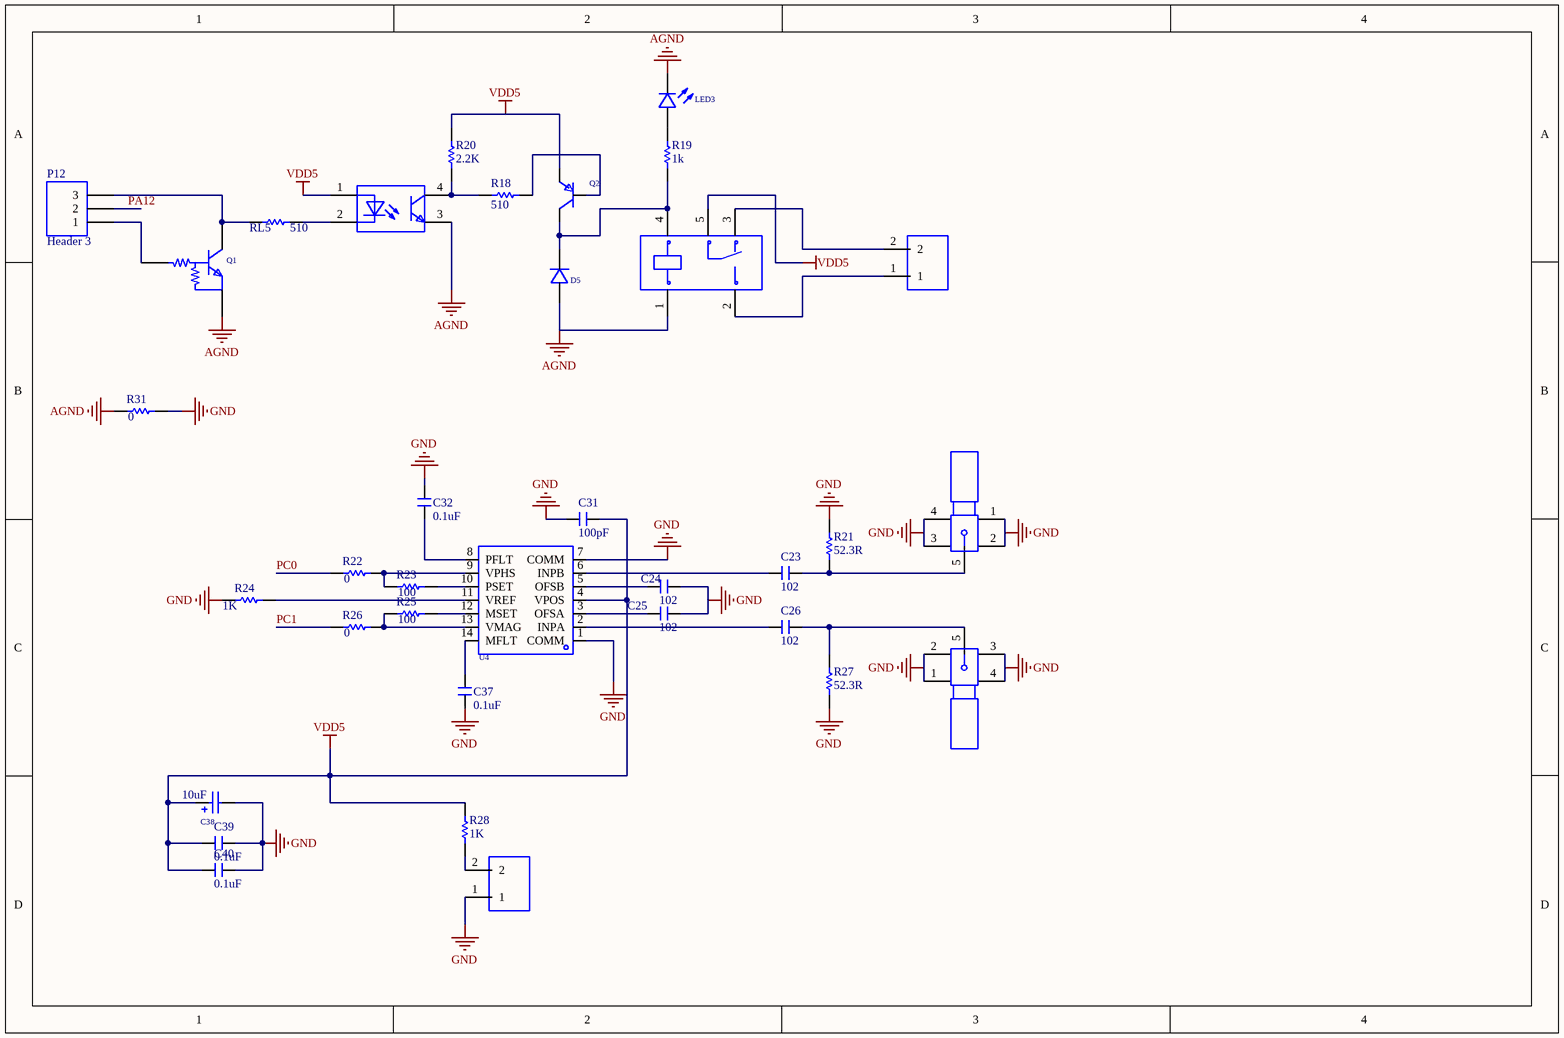
[diagram p0: MISC51485-4.schdoc]
# Altium project MISC51485-2.PrjPcb (part 1 of 2)
2 sheets, 98 parts. Net scope: global (net labels, ports and power ports of the same name join across sheets).
Board file: MISC51485.pcbdoc
Sheets:
  MISC51485-4.schdoc
  MISC51485-3.schdoc

## Sheet MISC51485-4.schdoc
size 292 x 193 mm; Device: *_1; SheetNumber: 2; SheetTotal: 2; Name: MISC51485

### Parts
C23  102  [C0603]
C24  102  [C0603]
C25  102  [C0603]
C26  102  [C0603]
C31  100pF  [C0603]
C32  0.1uF  [C0603]
C37  0.1uF  [C0603]
C38  10uF  [CAP-SMD_L3.2-W1.6-RD-C7171]
C39  0.1uF  [C0603]
C40  0.1uF  [C0603]
D5  1N4007W  [SOD-123FL_L2.7-W1.8-LS3.8-RD]  (value not drawn)
LED3  NCD0603R1_C84263  [LED0603-RD_RED]  (value not drawn)
P12  Header 3  [HDR1X3]
P13  WJ126V-5.0-2P  [CONN-TH_WJ126V-5.0-2P]  (value not drawn)
P17  WJ126V-5.0-2P  [CONN-TH_WJ126V-5.0-2P]  (value not drawn)
Q1  DTC143ECA  [SOT-23-3_L2.9-W1.6-P1.90-LS2.8-BR]  (value not drawn)
Q2  MMBT3906  [SOT-23-3_L2.9-W1.3-P1.90-LS2.4-BR]  (value not drawn)
R18  10k  [R0603 - duplicate]  (value not drawn)
R19  10k  [R0603 - duplicate]  (value not drawn)
R20  10k  [R0603 - duplicate]  (value not drawn)
R21  52.3R  [R0603]
R22  0  [R0603]
R23  100  [R0603]
R24  1K  [R0603]
R25  100  [R0603]
R26  0  [R0603]
R27  52.3R  [R0603]
R28  1K  [R0603]
R31  0  [R0603]
RF1  BWSMA-KWE-Z001  [SMA-TH_BWSMA-KWE-Z001]  (value not drawn)
RF?1  BWSMA-KWE-Z001  [SMA-TH_BWSMA-KWE-Z001]  (value not drawn)
RL5  330  [R0603 - duplicate]  (value not drawn)
RLY1  SRD-05VDC-SL-C  [RELAY-TH_SRD-XXVDC-XL-C]  (value not drawn)
U4  AD8302ARUZ-RL7  [TSSOP-14_L5.0-W4.4-P0.65-LS6.4-BL]  (value not drawn)
U6  BPC-817SC  [OPTO-SMD-4_L4.6-W6.5-P2.54-LS10.3-BR]  (value not drawn)

### Nets
AGND: D5.2(A) LED3.1(K) Q1.2(E) R31.1 RLY1.1 U6.3
GND: C24.1 C25.1 C31.2 C32.2 C37.1 C38.2 C39.1 C40.1 P17.1 R21.2 R24.1 R27.1 R31.2 RF1.1 RF1.2 RF1.3 RF1.4 RF?1.1 RF?1.2 RF?1.3 RF?1.4 U4.1(COMM) U4.7(COMM)
VDD5: C31.1 C38.1 C39.2 C40.2 Q2.2(E) R20.1 R28.2 RLY1.5 U4.4(VPOS) U6.1
PA12: P12.2
PC0: R22.1
PC1: R26.1
NetC23_1: C23.1 R21.1 RF1.5
NetC23_2: C23.2 U4.6(INPB)
NetC24_2: C24.2 U4.5(OFSB)
NetC25_2: C25.2 U4.3(OFSA)
NetC26_1: C26.1 R27.2 RF?1.5
NetC26_2: C26.2 U4.2(INPA)
NetC32_1: C32.1 U4.8(PFLT)
NetC37_2: C37.2 U4.14(MFLT)
NetD5_1: D5.1(K) Q2.3(C) R19.2 RLY1.4
NetLED3_2: LED3.2(A) R19.1
NetP12_1: P12.1 Q1.1(B)
NetP12_3: P12.3 Q1.3(C) RL5.1
NetP13_1: P13.1 RLY1.2
NetP13_2: P13.2 RLY1.3
NetP17_2: P17.2 R28.1
NetQ2_1: Q2.1(B) R18.2
NetR18_1: R18.1 R20.2 U6.4
NetR22_2: R22.2 R23.1 U4.9(VPHS)
NetR23_2: R23.2 U4.10(PSET)
NetR24_2: R24.2 U4.11(VREF)
NetR25_1: R25.1 R26.2 U4.13(VMAG)
NetR25_2: R25.2 U4.12(MSET)
NetRL5_2: RL5.2 U6.2

### Library data of the parts
C23 = 102: BOM名称: 无极性贴片电容; Origin Footprint: C 0201_L; OriginFootprint 2: C 0402_L; OriginFootprint 3: C 0603_L; OriginFootprint 4: C 0805_L; OriginFootprint 5: C 1206_L; OriginFootprint 6: C 1210_L; OriginFootprint 7: C 1808_L; OriginFootprint 8: C 1812_L; OriginFootprint 9: C 1825_L; OriginFootprint 10: C 2225_L; OriginFootprint 11: C 0201_M; OriginFootprint 12: C 0402_M; OriginFootprint 13: C 0603_M; OriginFootprint 14: C 0805_M; OriginFootprint 15: C 1206_M; OriginFootprint 16: C 1210_M; OriginFootprint 17: C 1808_M; OriginFootprint 18: C 1812_M; OriginFootprint 19: C 1825_M; OriginFootprint 20: C 2225_M; UniqueId: a6f4b5c625a68d3b; SymbolName: C; AddInBom: yes; ModelId: fca5be93b99f4b5a9a2fd372d58c31d9; Device: 102; DesignItemID: C; LibraryName: 3.1   - 电阻-电容-电感; Description: 102; FootprintName: C0603; ModelName: C0603
C24 = 102: BOM名称: 无极性贴片电容; Origin Footprint: C 0201_L; OriginFootprint 2: C 0402_L; OriginFootprint 3: C 0603_L; OriginFootprint 4: C 0805_L; OriginFootprint 5: C 1206_L; OriginFootprint 6: C 1210_L; OriginFootprint 7: C 1808_L; OriginFootprint 8: C 1812_L; OriginFootprint 9: C 1825_L; OriginFootprint 10: C 2225_L; OriginFootprint 11: C 0201_M; OriginFootprint 12: C 0402_M; OriginFootprint 13: C 0603_M; OriginFootprint 14: C 0805_M; OriginFootprint 15: C 1206_M; OriginFootprint 16: C 1210_M; OriginFootprint 17: C 1808_M; OriginFootprint 18: C 1812_M; OriginFootprint 19: C 1825_M; OriginFootprint 20: C 2225_M; UniqueId: 8647aab959e5cc85; SymbolName: C; AddInBom: yes; ModelId: fca5be93b99f4b5a9a2fd372d58c31d9; Device: 102; DesignItemID: C; LibraryName: 3.1   - 电阻-电容-电感; Description: 102; FootprintName: C0603; ModelName: C0603
C25 = 102: BOM名称: 无极性贴片电容; Origin Footprint: C 0201_L; OriginFootprint 2: C 0402_L; OriginFootprint 3: C 0603_L; OriginFootprint 4: C 0805_L; OriginFootprint 5: C 1206_L; OriginFootprint 6: C 1210_L; OriginFootprint 7: C 1808_L; OriginFootprint 8: C 1812_L; OriginFootprint 9: C 1825_L; OriginFootprint 10: C 2225_L; OriginFootprint 11: C 0201_M; OriginFootprint 12: C 0402_M; OriginFootprint 13: C 0603_M; OriginFootprint 14: C 0805_M; OriginFootprint 15: C 1206_M; OriginFootprint 16: C 1210_M; OriginFootprint 17: C 1808_M; OriginFootprint 18: C 1812_M; OriginFootprint 19: C 1825_M; OriginFootprint 20: C 2225_M; UniqueId: 67f8b94986dc5590; SymbolName: C; AddInBom: yes; ModelId: fca5be93b99f4b5a9a2fd372d58c31d9; Device: 102; DesignItemID: C; LibraryName: 3.1   - 电阻-电容-电感; Description: 102; FootprintName: C0603; ModelName: C0603
C26 = 102: BOM名称: 无极性贴片电容; Origin Footprint: C 0201_L; OriginFootprint 2: C 0402_L; OriginFootprint 3: C 0603_L; OriginFootprint 4: C 0805_L; OriginFootprint 5: C 1206_L; OriginFootprint 6: C 1210_L; OriginFootprint 7: C 1808_L; OriginFootprint 8: C 1812_L; OriginFootprint 9: C 1825_L; OriginFootprint 10: C 2225_L; OriginFootprint 11: C 0201_M; OriginFootprint 12: C 0402_M; OriginFootprint 13: C 0603_M; OriginFootprint 14: C 0805_M; OriginFootprint 15: C 1206_M; OriginFootprint 16: C 1210_M; OriginFootprint 17: C 1808_M; OriginFootprint 18: C 1812_M; OriginFootprint 19: C 1825_M; OriginFootprint 20: C 2225_M; UniqueId: 008a446d5bfc6874; SymbolName: C; AddInBom: yes; ModelId: fca5be93b99f4b5a9a2fd372d58c31d9; Device: 102; DesignItemID: C; LibraryName: 3.1   - 电阻-电容-电感; Description: 102; FootprintName: C0603; ModelName: C0603
C31 = 100pF: BOM名称: 无极性贴片电容; Origin Footprint: C 0201_L; OriginFootprint 2: C 0402_L; OriginFootprint 3: C 0603_L; OriginFootprint 4: C 0805_L; OriginFootprint 5: C 1206_L; OriginFootprint 6: C 1210_L; OriginFootprint 7: C 1808_L; OriginFootprint 8: C 1812_L; OriginFootprint 9: C 1825_L; OriginFootprint 10: C 2225_L; OriginFootprint 11: C 0201_M; OriginFootprint 12: C 0402_M; OriginFootprint 13: C 0603_M; OriginFootprint 14: C 0805_M; OriginFootprint 15: C 1206_M; OriginFootprint 16: C 1210_M; OriginFootprint 17: C 1808_M; OriginFootprint 18: C 1812_M; OriginFootprint 19: C 1825_M; OriginFootprint 20: C 2225_M; UniqueId: 7237750993165679; SymbolName: C; AddInBom: yes; ModelId: fca5be93b99f4b5a9a2fd372d58c31d9; Device: 100pF; DesignItemID: C; LibraryName: 3.1   - 电阻-电容-电感; Description: 100pF; FootprintName: C0603; ModelName: C0603
C32 = 0.1uF: BOM名称: 无极性贴片电容; Origin Footprint: C 0201_L; OriginFootprint 2: C 0402_L; OriginFootprint 3: C 0603_L; OriginFootprint 4: C 0805_L; OriginFootprint 5: C 1206_L; OriginFootprint 6: C 1210_L; OriginFootprint 7: C 1808_L; OriginFootprint 8: C 1812_L; OriginFootprint 9: C 1825_L; OriginFootprint 10: C 2225_L; OriginFootprint 11: C 0201_M; OriginFootprint 12: C 0402_M; OriginFootprint 13: C 0603_M; OriginFootprint 14: C 0805_M; OriginFootprint 15: C 1206_M; OriginFootprint 16: C 1210_M; OriginFootprint 17: C 1808_M; OriginFootprint 18: C 1812_M; OriginFootprint 19: C 1825_M; OriginFootprint 20: C 2225_M; UniqueId: b3514bd818d3e114; SymbolName: C; AddInBom: yes; ModelId: fca5be93b99f4b5a9a2fd372d58c31d9; Device: 0.1uF; DesignItemID: C; LibraryName: 3.1   - 电阻-电容-电感; Description: 0.1uF; FootprintName: C0603; ModelName: C0603
C37 = 0.1uF: BOM名称: 无极性贴片电容; Origin Footprint: C 0201_L; OriginFootprint 2: C 0402_L; OriginFootprint 3: C 0603_L; OriginFootprint 4: C 0805_L; OriginFootprint 5: C 1206_L; OriginFootprint 6: C 1210_L; OriginFootprint 7: C 1808_L; OriginFootprint 8: C 1812_L; OriginFootprint 9: C 1825_L; OriginFootprint 10: C 2225_L; OriginFootprint 11: C 0201_M; OriginFootprint 12: C 0402_M; OriginFootprint 13: C 0603_M; OriginFootprint 14: C 0805_M; OriginFootprint 15: C 1206_M; OriginFootprint 16: C 1210_M; OriginFootprint 17: C 1808_M; OriginFootprint 18: C 1812_M; OriginFootprint 19: C 1825_M; OriginFootprint 20: C 2225_M; UniqueId: ab97e3f8b5f3b4a6; SymbolName: C; AddInBom: yes; ModelId: fca5be93b99f4b5a9a2fd372d58c31d9; Device: 0.1uF; DesignItemID: C; LibraryName: 3.1   - 电阻-电容-电感; Description: 0.1uF; FootprintName: C0603; ModelName: C0603
C38 = 10uF_1: Manufacturer: Kyocera AVX; Manufacturer Part: TAJA106K016RNJ; Add into BOM: yes; Tolerance: ±10%; Rated Voltage: 16V; Equivalent Series Resistance(ESR): 3Ω@100kHz; UniqueId: da7f3e643a6c899d; SymbolName: 10uF钽电容; Device: 10uF_1; LCSC Part Name: 10uF ±10% 16V; Supplier Part: C7171; Supplier Footprint: CASE-A-3216; JLCPCB Part Class: Basic Part; Datasheet: https://atta.szlcsc.com/upload/public/pdf/source/20160107/1457707750344.pdf; Supplier: LCSC; Convert to PCB: yes; Value: 10uF; Operating Temperature: -55℃~+125℃; DesignItemID: 10uF钽电容; LibraryName: Schlib1; Description: 10uF; FootprintName: CAP-SMD_L3.2-W1.6-RD-C7171
C39 = 0.1uF: BOM名称: 无极性贴片电容; Origin Footprint: C 0201_L; OriginFootprint 2: C 0402_L; OriginFootprint 3: C 0603_L; OriginFootprint 4: C 0805_L; OriginFootprint 5: C 1206_L; OriginFootprint 6: C 1210_L; OriginFootprint 7: C 1808_L; OriginFootprint 8: C 1812_L; OriginFootprint 9: C 1825_L; OriginFootprint 10: C 2225_L; OriginFootprint 11: C 0201_M; OriginFootprint 12: C 0402_M; OriginFootprint 13: C 0603_M; OriginFootprint 14: C 0805_M; OriginFootprint 15: C 1206_M; OriginFootprint 16: C 1210_M; OriginFootprint 17: C 1808_M; OriginFootprint 18: C 1812_M; OriginFootprint 19: C 1825_M; OriginFootprint 20: C 2225_M; UniqueId: 149c9a252617316b; SymbolName: C; AddInBom: yes; ModelId: fca5be93b99f4b5a9a2fd372d58c31d9; Device: 0.1uF; DesignItemID: C; LibraryName: 3.1   - 电阻-电容-电感; Description: 0.1uF; FootprintName: C0603; ModelName: C0603
C40 = 0.1uF: BOM名称: 无极性贴片电容; Origin Footprint: C 0201_L; OriginFootprint 2: C 0402_L; OriginFootprint 3: C 0603_L; OriginFootprint 4: C 0805_L; OriginFootprint 5: C 1206_L; OriginFootprint 6: C 1210_L; OriginFootprint 7: C 1808_L; OriginFootprint 8: C 1812_L; OriginFootprint 9: C 1825_L; OriginFootprint 10: C 2225_L; OriginFootprint 11: C 0201_M; OriginFootprint 12: C 0402_M; OriginFootprint 13: C 0603_M; OriginFootprint 14: C 0805_M; OriginFootprint 15: C 1206_M; OriginFootprint 16: C 1210_M; OriginFootprint 17: C 1808_M; OriginFootprint 18: C 1812_M; OriginFootprint 19: C 1825_M; OriginFootprint 20: C 2225_M; UniqueId: 67c6b1130f95bc58; SymbolName: C; AddInBom: yes; ModelId: fca5be93b99f4b5a9a2fd372d58c31d9; Device: 0.1uF; DesignItemID: C; LibraryName: 3.1   - 电阻-电容-电感; Description: 0.1uF; FootprintName: C0603; ModelName: C0603
D5 = 1N4007W: Manufacturer: 宏迦橙; Add into BOM: yes; Diode Configuration: 独立式; Forward Voltage (Vf@If): 1V@1.0A; Reverse Voltage (Vr): 1kV; Rectified Current: 1A; Reverse Leakage Current (Ir): 2uA@1000V; UniqueId: f6a2299b727f22e5; SymbolName: 1N4007W_C18199088; Device: 1N4007W; LCSC Part Name: 1N4007W; Supplier Part: C18199088; Manufacturer Part: 1N4007W; Supplier Footprint: SOD-123FL; JLCPCB Part Class: Extended Part; Datasheet: https://atta.szlcsc.com/upload/public/pdf/source/20230925/B0AB2B510D392D7083D021E804ED238F.pdf; Supplier: LCSC; Convert to PCB: yes; DesignItemID: 1N4007W_C18199088; LibraryName: Schlib1; FootprintName: SOD-123FL_L2.7-W1.8-LS3.8-RD
LED3 = NCD0603R1_C84263: Manufacturer: 国星光电; Add into BOM: yes; Emitted Color: 红灯; UniqueId: 01e448f2d6732d04; ModelId: 74041d3a270d435c8600a9ab9b7641c0; Device: NCD0603R1_C84263; LCSC Part Name: 红灯; Supplier Part: C84263; Manufacturer Part: NCD0603R1; Supplier Footprint: 0603; JLCPCB Part Class: Extended Part; Datasheet: https://atta.szlcsc.com/upload/public/pdf/source/20200820/C84263_DABC6A75E58F576973B407FDBA283D60.pdf; Supplier: LCSC; Convert to PCB: yes; DesignItemID: NCD0603R1_C84263; LibraryName: Schlib1; SymbolName: NCD0603R1_C84263; FootprintName: LED0603-RD_RED; ModelName: LED0603-RD_RED
P12 = Header 3: Header, 3-Pin; UniqueId: 7119f1a9b2ee76bc; AddInBom: yes; Device: Header 3; LatestRevisionDate: 17-Jul-2002; LatestRevisionNote: Re-released for DXP Platform.; DesignItemID: Header 3; LibraryName: Miscellaneous Connectors; SymbolName: Header 3; FootprintName: HDR1X3; Publisher: Altium Limited
P13 = WJ126V-5.0-2P_1: Manufacturer: KANGNEX(康奈克斯电气); Add into BOM: yes; Structure: 1x2P; Pitch: 5mm; Current Rating (Max): 18A; Voltage Rating (Max): 250V; Wire Gauge - AWG: 14~26; Wire Gauge - mm2: 2.5; Number of PINs Per Row: 2; UniqueId: 24d56ee73e068b48; SymbolName: 螺钉接线端子; Device: WJ126V-5.0-2P_1; Supplier: LCSC; Manufacturer Part: WJ126V-5.0-2P; Supplier Part: C8404; JLCPCB Part Class: Extended Part; LCSC Part Name: 5mm 1x2P 排数:1 每排P数:2 直插; Supplier Footprint: 插件,P=5mm; Datasheet: https://atta.szlcsc.com/upload/public/pdf/source/20191225/C8404_8F52D87DF851D149A4DEA9BD9FA83F9A.pdf; Convert to PCB: yes; Color: 绿色; Mounting Style: 直插; Number of Pins: 2P; Number of Rows: 1; Operating Temperature Range: -40℃~+105℃; DesignItemID: 螺钉接线端子; LibraryName: Schlib1; FootprintName: CONN-TH_WJ126V-5.0-2P
P17 = WJ126V-5.0-2P_1: Manufacturer: KANGNEX(康奈克斯电气); Add into BOM: yes; Structure: 1x2P; Pitch: 5mm; Current Rating (Max): 18A; Voltage Rating (Max): 250V; Wire Gauge - AWG: 14~26; Wire Gauge - mm2: 2.5; Number of PINs Per Row: 2; UniqueId: e8b683bff28da981; SymbolName: 螺钉接线端子; Device: WJ126V-5.0-2P_1; Supplier: LCSC; Manufacturer Part: WJ126V-5.0-2P; Supplier Part: C8404; JLCPCB Part Class: Extended Part; LCSC Part Name: 5mm 1x2P 排数:1 每排P数:2 直插; Supplier Footprint: 插件,P=5mm; Datasheet: https://atta.szlcsc.com/upload/public/pdf/source/20191225/C8404_8F52D87DF851D149A4DEA9BD9FA83F9A.pdf; Convert to PCB: yes; Color: 绿色; Mounting Style: 直插; Number of Pins: 2P; Number of Rows: 1; Operating Temperature Range: -40℃~+105℃; DesignItemID: 螺钉接线端子; LibraryName: Schlib1; FootprintName: CONN-TH_WJ126V-5.0-2P
Q1 = DTC143ECA: Manufacturer: CJ(江苏长电/长晶); Add into BOM: yes; Collector-Emitter Breakdown Voltage (Vceo): 50V; Collector Current (Ic): 100mA; Power Dissipation (Pd): 200mW; UniqueId: 047b734180970fea; Device: DTC143ECA; LCSC Part Name: 耐压:50V 电流:100mA; Supplier Part: C13871; Manufacturer Part: DTC143ECA; Supplier Footprint: SOT-23; JLCPCB Part Class: Extended Part; Datasheet: https://atta.szlcsc.com/upload/public/pdf/source/20140809/1457707204735.pdf; Supplier: LCSC; Convert to PCB: yes; Transistor Type: -; DesignItemID: DTC143ECA; LibraryName: ALLSchlib; SymbolName: DTC143ECA; FootprintName: SOT-23-3_L2.9-W1.6-P1.90-LS2.8-BR
Q2 = MMBT3906: Manufacturer: ST(先科); Add into BOM: yes; Transistor Type: PNP; Collector Current (Ic): 200mA; Collector-Emitter Breakdown Voltage (Vceo): 40V; Power Dissipation (Pd): 350mW; DC Current Gain (hFE@Ic,Vce): 100@10mA,1V; Transition Frequency (fT): 250MHz; Collector Cut-Off Current (Icbo): 50nA; Collector-Emitter Saturation Voltage (VCE(sat)@Ic,Ib): 400mV@50mA,5mA; UniqueId: 4adba29ee04e5395; SymbolName: MMBT3906_C84105; Device: MMBT3906; LCSC Part Name: PNP 电流:200mA 耐压:40V; Supplier Part: C84105; Manufacturer Part: MMBT3906; Supplier Footprint: SOT-23; JLCPCB Part Class: Extended Part; Datasheet: https://atta.szlcsc.com/upload/public/pdf/source/20161024/1477288599957.pdf; Supplier: LCSC; Convert to PCB: yes; Operating Temperature: -; DesignItemID: MMBT3906_C84105; LibraryName: ALLSchlib; FootprintName: SOT-23-3_L2.9-W1.3-P1.90-LS2.4-BR
R18 = 10k_1: Res; Origin Footprint: RES[0805]; OriginFootprint 3: RES[0603]; UniqueId: 1bd7cdeea74e381f; AddInBom: yes; Device: 10k_1; OriginFootprint 2: Res; DesignItemID: Res; LibraryName: Sean; SymbolName: Res; FootprintName: R0603 - duplicate
R19 = 10k_1: Res; Origin Footprint: RES[0805]; OriginFootprint 3: RES[0603]; UniqueId: 2e979fad964ca14d; AddInBom: yes; Device: 10k_1; OriginFootprint 2: Res; DesignItemID: Res; LibraryName: Sean; SymbolName: Res; FootprintName: R0603 - duplicate
R20 = 10k_1: Res; Origin Footprint: RES[0805]; OriginFootprint 3: RES[0603]; UniqueId: 237b6fcbd18a81e0; AddInBom: yes; Device: 10k_1; OriginFootprint 2: Res; DesignItemID: Res; LibraryName: Sean; SymbolName: Res; FootprintName: R0603 - duplicate
R21 = 52.3R: Origin Footprint: RES[0805]; OriginFootprint 2: Res; UniqueId: c67641ae573ea1fc; AddInBom: yes; ModelId: fc143cca1e79419f9cd78b61e9279f08; Device: 52.3R; DesignItemID: Res; LibraryName: Sean; Description: 52.3R; SymbolName: Res; FootprintName: R0603; ModelName: R0603
R22 = 0: Origin Footprint: RES[0805]; OriginFootprint 2: Res; UniqueId: c805ee3f93c0e373; AddInBom: yes; ModelId: fc143cca1e79419f9cd78b61e9279f08; Device: 0; DesignItemID: Res; LibraryName: Sean; Description: 0; SymbolName: Res; FootprintName: R0603; ModelName: R0603
R23 = 100: Origin Footprint: RES[0805]; OriginFootprint 2: Res; UniqueId: d677bbbfc70c791c; AddInBom: yes; ModelId: fc143cca1e79419f9cd78b61e9279f08; Device: 100; DesignItemID: Res; LibraryName: Sean; Description: 100; SymbolName: Res; FootprintName: R0603; ModelName: R0603
R24 = 1K: Origin Footprint: RES[0805]; OriginFootprint 2: Res; UniqueId: a5af7fcca697766d; AddInBom: yes; ModelId: fc143cca1e79419f9cd78b61e9279f08; Device: 1K; DesignItemID: Res; LibraryName: Sean; Description: 1K; SymbolName: Res; FootprintName: R0603; ModelName: R0603
R25 = 100: Origin Footprint: RES[0805]; OriginFootprint 2: Res; UniqueId: cf753b156485d875; AddInBom: yes; ModelId: fc143cca1e79419f9cd78b61e9279f08; Device: 100; DesignItemID: Res; LibraryName: Sean; Description: 100; SymbolName: Res; FootprintName: R0603; ModelName: R0603
R26 = 0: Origin Footprint: RES[0805]; OriginFootprint 2: Res; UniqueId: c4d44f1d54239503; AddInBom: yes; ModelId: fc143cca1e79419f9cd78b61e9279f08; Device: 0; DesignItemID: Res; LibraryName: Sean; Description: 0; SymbolName: Res; FootprintName: R0603; ModelName: R0603
R27 = 52.3R: Origin Footprint: RES[0805]; OriginFootprint 2: Res; UniqueId: ca1ef6058e20807c; AddInBom: yes; ModelId: fc143cca1e79419f9cd78b61e9279f08; Device: 52.3R; DesignItemID: Res; LibraryName: Sean; Description: 52.3R; SymbolName: Res; FootprintName: R0603; ModelName: R0603
R28 = 1K: Origin Footprint: RES[0805]; OriginFootprint 2: Res; UniqueId: 8d3fec937682270b; AddInBom: yes; ModelId: fc143cca1e79419f9cd78b61e9279f08; Device: 1K; DesignItemID: Res; LibraryName: Sean; Description: 1K; SymbolName: Res; FootprintName: R0603; ModelName: R0603
R31 = 0: Origin Footprint: RES[0805]; OriginFootprint 2: Res; UniqueId: ecc590771c67343e; AddInBom: yes; ModelId: fc143cca1e79419f9cd78b61e9279f08; Device: 0; DesignItemID: Res; LibraryName: Sean; Description: 0; SymbolName: Res; FootprintName: R0603; ModelName: R0603
RF1 = BWSMA-KWE-Z001_1: Manufacturer: BAT WIRELESS(蝙蝠无线); Add into BOM: yes; Connector Type: 板端; Interface Type: 内孔; Number of Ports: 1; Interface Diameter: 5.3mm; RF Series: SMA; Impedance: 50Ω; Style: 弯头; UniqueId: 5065ca7df19ad891; Device: BWSMA-KWE-Z001_1; Supplier: LCSC; Supplier Part: C496551; Manufacturer Part: BWSMA-KWE-Z001; JLCPCB Part Class: Extended Part; LCSC Part Name: 内孔 SMA 弯头; Supplier Footprint: 插件; Datasheet: https://atta.szlcsc.com/upload/public/pdf/source/20231017/997A8C2ADA7F8034A89BE1264F38CE52.pdf; Convert to PCB: yes; Interface Length/Height: -; Frequency-Max: -; Contact Material: -; Contact Plating: -; Operating Temperature Range: -; Soldering Temperature(Max): -; DesignItemID: BWSMA-KWE-Z001; LibraryName: Schlib1; SymbolName: BWSMA-KWE-Z001; FootprintName: SMA-TH_BWSMA-KWE-Z001
RF?1 = BWSMA-KWE-Z001: Manufacturer: BAT WIRELESS(蝙蝠无线); Add into BOM: yes; Connector Type: 板端; Interface Type: 内孔; Number of Ports: 1; Interface Diameter: 5.3mm; RF Series: SMA; Impedance: 50Ω; Style: 弯头; UniqueId: 7768e29b96b67243; Device: BWSMA-KWE-Z001; Supplier: LCSC; Supplier Part: C496551; Manufacturer Part: BWSMA-KWE-Z001; JLCPCB Part Class: Extended Part; LCSC Part Name: 内孔 SMA 弯头; Supplier Footprint: 插件; Datasheet: https://atta.szlcsc.com/upload/public/pdf/source/20231017/997A8C2ADA7F8034A89BE1264F38CE52.pdf; Convert to PCB: yes; Interface Length/Height: -; Frequency-Max: -; Contact Material: -; Contact Plating: -; Operating Temperature Range: -; Soldering Temperature(Max): -; DesignItemID: BWSMA-KWE-Z001; LibraryName: Schlib1; SymbolName: BWSMA-KWE-Z001; FootprintName: SMA-TH_BWSMA-KWE-Z001
RL5 = 330: Res; Origin Footprint: RES[0805]; OriginFootprint 3: RES[0603]; UniqueId: 4e5f24055ba3677c; AddInBom: yes; Device: 330; OriginFootprint 2: Res; DesignItemID: Res; LibraryName: Sean; SymbolName: Res; FootprintName: R0603 - duplicate
RLY1 = SRD-05VDC-SL-C: Manufacturer: 松乐; Add into BOM: yes; Coil Voltage: 5V; Contact Form: 一组转换:1C(单刀双掷-转换); Pin Number: 5; Maximum Switching Voltage: 250V@AC; Coil Rated Power: 360mW; Maximum Switching Current: 15A; Coil Type: 无极性-单线圈; Coil Resistance: 70Ω; Contact Resistance: 100mΩ; Operate Time: 10ms; UniqueId: 1294ab66729aac8a; Device: SRD-05VDC-SL-C; LCSC Part Name: 蓝色; Supplier Part: C35449; Manufacturer Part: SRD-05VDC-SL-C; Supplier Footprint: 插件,15.6x19.2mm; JLCPCB Part Class: Extended Part; Datasheet: https://atta.szlcsc.com/upload/public/pdf/source/20200305/C490149_C96E4098A3B1FFB377D5AD2E40B7C2A8.pdf; Supplier: LCSC; Convert to PCB: yes; Contact Rating: -; Release Time: 10ms; DesignItemID: SRD-05VDC-SL-C; LibraryName: Schlib1; SymbolName: SRD-05VDC-SL-C; FootprintName: RELAY-TH_SRD-XXVDC-XL-C
U4 = AD8302ARUZ-RL7: Manufacturer: ADI(亚德诺); Add into BOM: yes; Frequency Range: 2.7GHz; Input Range: -60dBm~0dBm; Supply Voltage: 2.7V~5.5V; Supply Current: 23mA; Accuracy: ±0.5dB; UniqueId: e5d1bee62801ccc5; Device: AD8302ARUZ-RL7; LCSC Part Name: RF/IF增益和相位检波器; Supplier Part: C408900; Manufacturer Part: AD8302ARUZ-RL7; Supplier Footprint: TSSOP-14; JLCPCB Part Class: Extended Part; Datasheet: https://atta.szlcsc.com/upload/public/pdf/source/20190807/C408900_5BB3D180A454BA6F4D99553AB0F529A5.pdf; Supplier: LCSC; Convert to PCB: yes; Applications: 通用; DesignItemID: AD8302ARUZ-RL7; LibraryName: Schlib1; SymbolName: AD8302ARUZ-RL7; FootprintName: TSSOP-14_L5.0-W4.4-P0.65-LS6.4-BL
U6 = BPC-817SC: Manufacturer: BrtLed(佰鸿); Add into BOM: yes; Input voltage type: DC; Output Type: 光电三极管; Voltage - Forward(Vf): 1.2V; Output Current: 50mA; Reverse Voltage: 6V; Load Voltage: 35V; Number of Outputs: 1; Vce Saturation(VCE(sat)): 100mV@1mA,20mA; Rise time: 4us@2mA,100Ω; Fall time: 3us@2mA,100Ω; UniqueId: cb0a5e759a2bc85d; Device: BPC-817SC; LCSC Part Name: DC输入; Supplier Part: C94736; Manufacturer Part: BPC-817SC; Supplier Footprint: SMD-4P; JLCPCB Part Class: Extended Part; Datasheet: https://atta.szlcsc.com/upload/public/pdf/source/20170228/1488267660599.pdf; Supplier: LCSC; Convert to PCB: yes; Operating Temperature: -40℃~+100℃; DesignItemID: BPC-817SC; LibraryName: Schlib1; SymbolName: BPC-817SC; FootprintName: OPTO-SMD-4_L4.6-W6.5-P2.54-LS10.3-BR

## Sheet MISC51485-3.schdoc: MISC51485
size 393 x 282 mm; SheetNumber: 1; SheetTotal: 2; Name: MISC51485
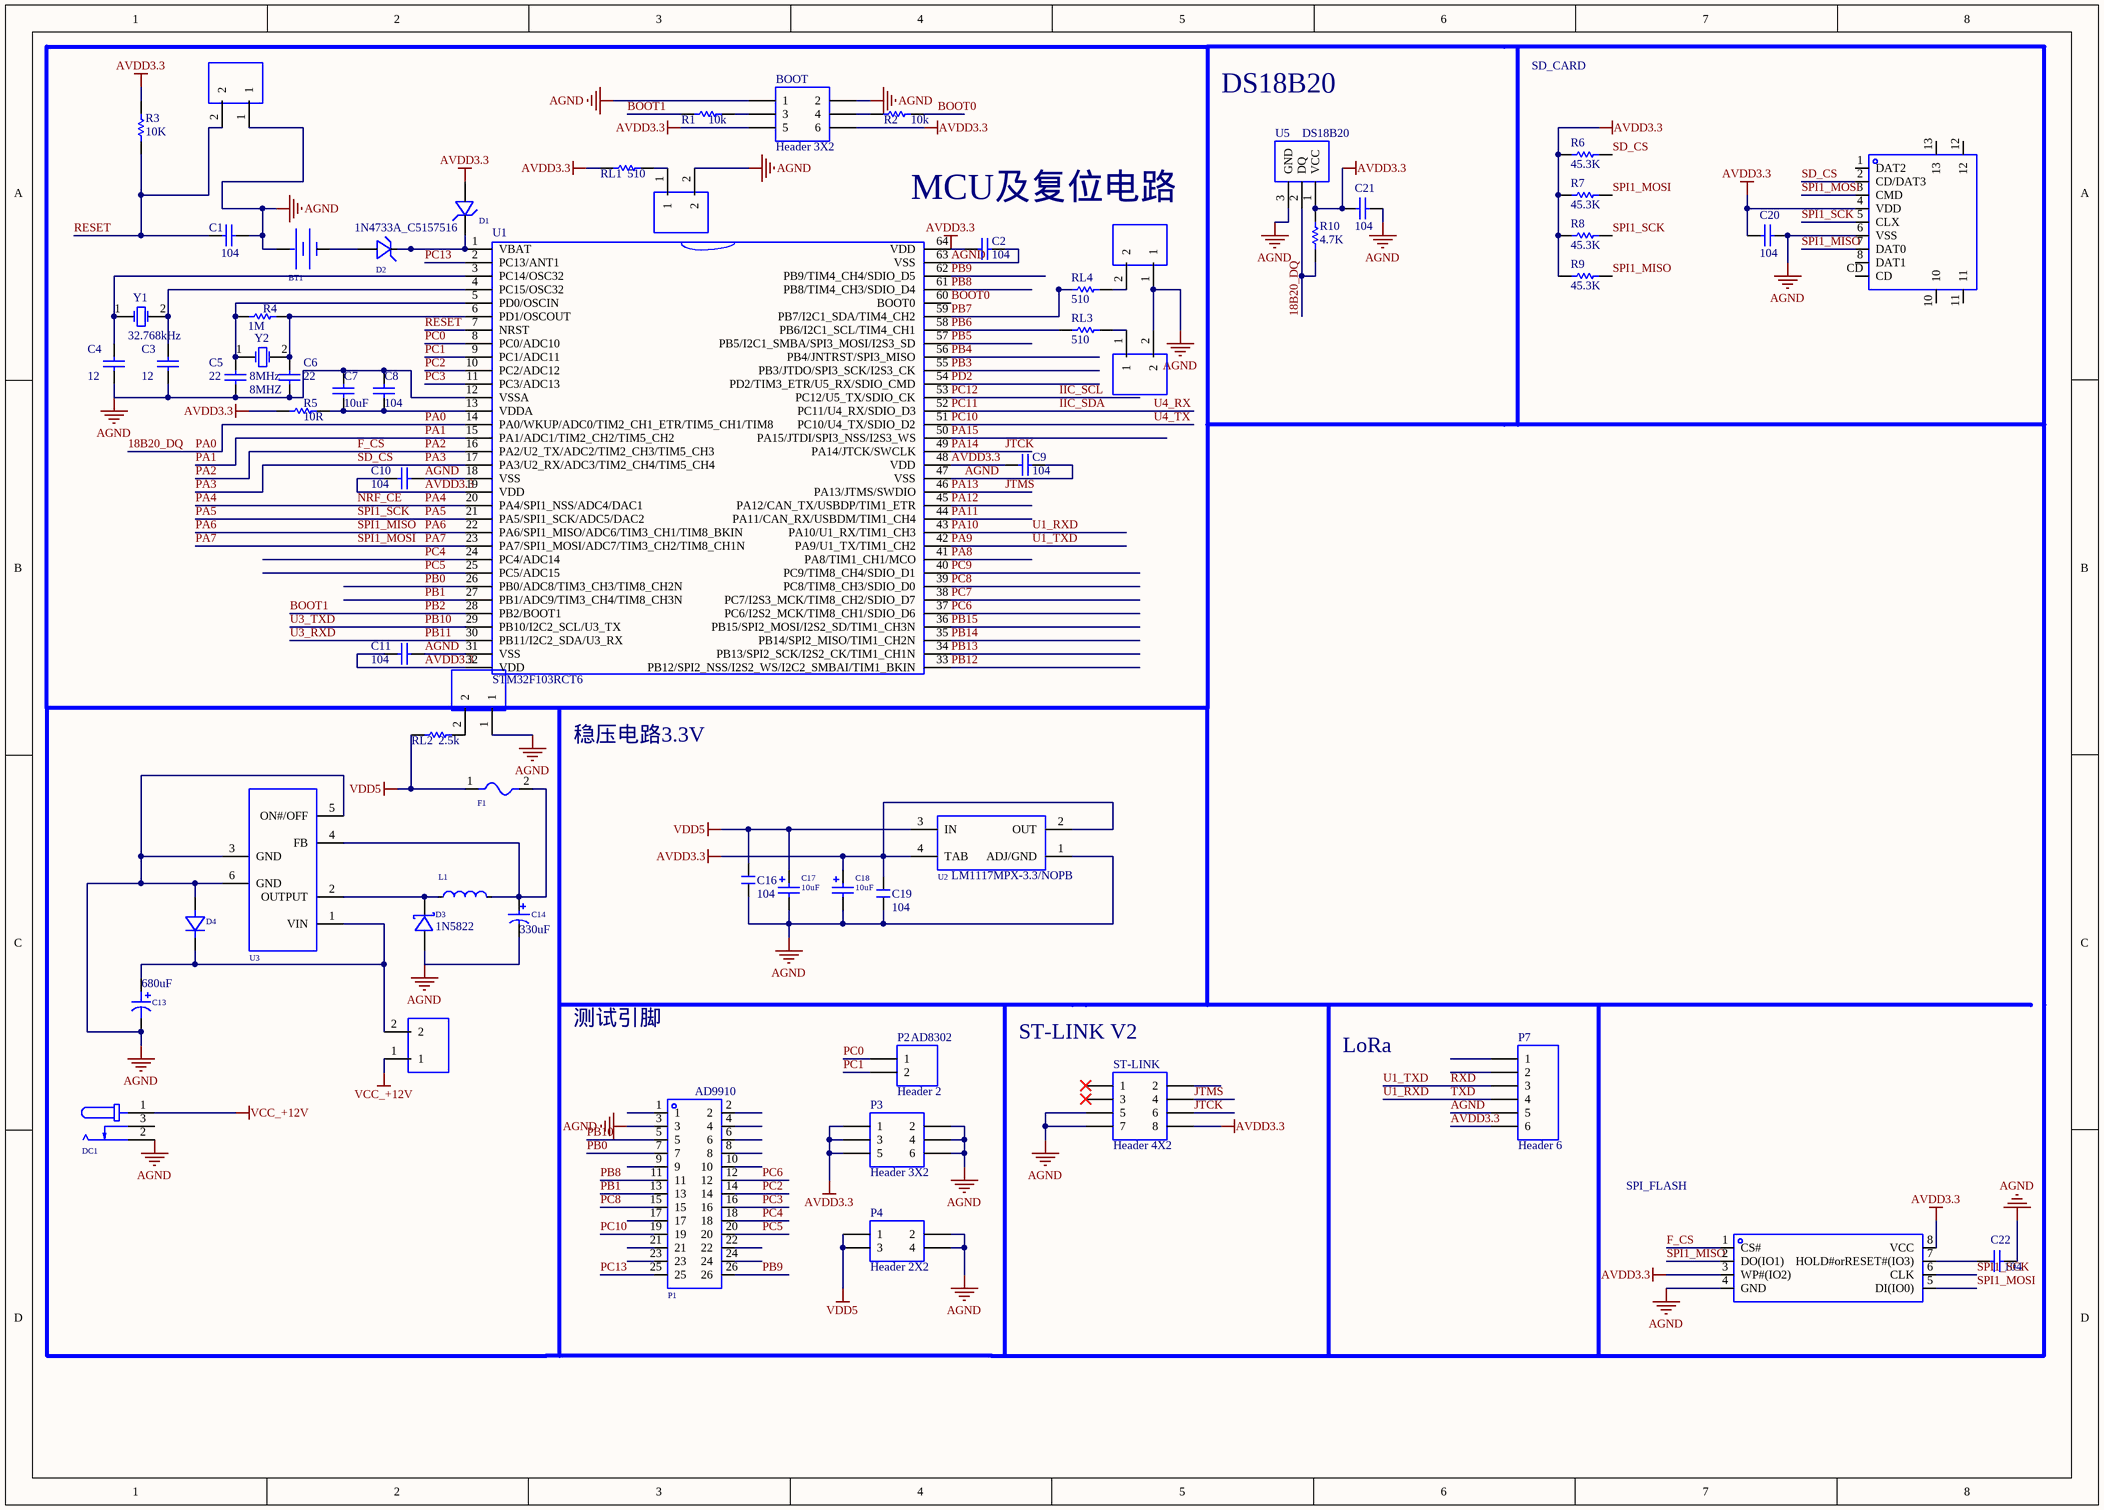
[diagram p1: MISC51485-3.schdoc]

### Parts
BOOT  Header 3X2  [HDR2X3]
BT1  BS-12-B3AA003  [BAT-SMD_BS-12-B3AA011]  (value not drawn)
C1  104  [C0603]
C2  104  [C0603]
C3  12pF  [C0603]  (value not drawn)
C4  12pF  [C0603]  (value not drawn)
C5  22pF  [C0603]  (value not drawn)
C6  22pF  [C0603]  (value not drawn)
C7  10uF  [C0603]
C8  104  [C0603]
C9  104  [C0603]
C10  104  [C0603]
C11  104  [C0603]
C13  GVM1V681M1010  [CAP-SMD_BD10.0-L10.3-W10.3-LS10.9-FD]  (value not drawn)
C14  EEEFK1V331P  [CAP-SMD_BD10.0-L10.3-W10.3-FD]  (value not drawn)
C16  104  [C0603]
C17  value 10uF  [CAP-SMD_L3.2-W1.6-RD-C7171]  (hidden comment: TAJA106K016RNJ)
C18  value 10uF  [CAP-SMD_L3.2-W1.6-RD-C7171]  (hidden comment: TAJA106K016RNJ)
C19  104  [C0603]
C20  Cap  [CAP[0603]]  (value not drawn)
C21  Cap  [CAP[0603]]  (value not drawn)
C22  Cap  [CAP[0603]]  (value not drawn)
CARD  TF PUSH  [TF-SMD_TF-PUSH]  (value not drawn)
D1  1N4733A_C5157516  [DO-41_BD2.4-L4.7-P8.70-D0.9-RD]  (value not drawn)
D2  1N4733A_C5157516  [DO-41_BD2.4-L4.7-P8.70-D0.9-RD]
D3  1N5822  [DO-201AD_BD5.3-L8.4-P12.50-D1.4-FD]
D4  1N4007_C727081  [SMA_L4.3-W2.5-LS5.0-RD]  (value not drawn)
DC1  DC-005-20A_C136744  [DC-IN-TH_DC-005-20A]  (value not drawn)
F1  BSMD1812-150-33V  [F1812]  (value not drawn)
L1  FXL0650-330-M  [IND-SMD_L7.0-W6.6_FXL0650]  (value not drawn)
P1  X1270WV-2x13A-6TV01  [IDC-TH_X1270WV-2X13A-6TV01]  (value not drawn)
P2  Header 2  [HDR1X2]
P3  Header 3X2  [HDR2X3]
P4  Header 2X2  [HDR2X2]
P7  Header 6  [HDR1X6]
P18  WJ126V-5.0-2P  [CONN-TH_WJ126V-5.0-2P]  (value not drawn)
P19  WJ126V-5.0-2P  [CONN-TH_WJ126V-5.0-2P]  (value not drawn)
P20  WJ126V-5.0-2P  [CONN-TH_WJ126V-5.0-2P]  (value not drawn)
P21  WJ126V-5.0-2P  [CONN-TH_WJ126V-5.0-2P]  (value not drawn)
P22  WJ126V-5.0-2P  [CONN-TH_WJ126V-5.0-2P]  (value not drawn)
P23  WJ126V-5.0-2P  [CONN-TH_WJ126V-5.0-2P]  (value not drawn)